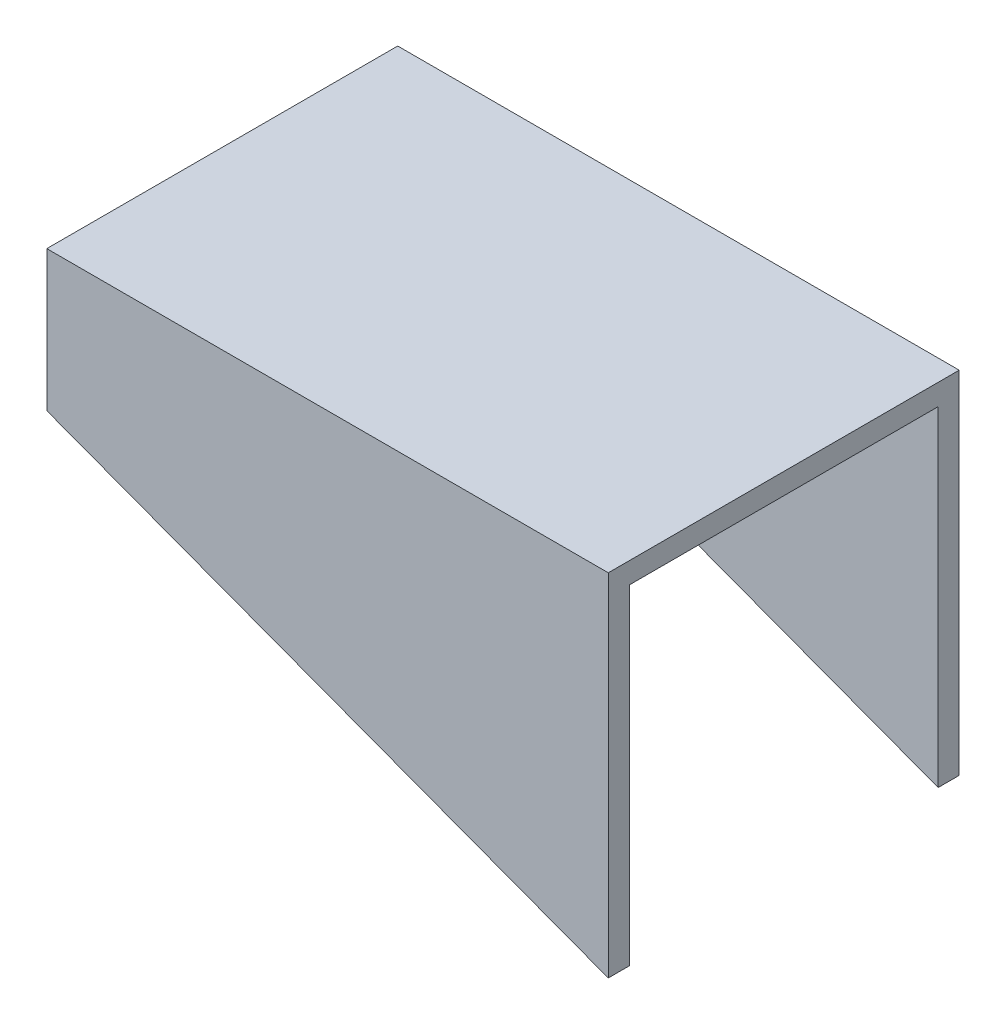
from build123d import *

# Parameters (mm, degrees)
EXTRUDE_1_DEPTH = 50
SHELL_1_T       = -3


with BuildPart() as part:
    # 草图1 → 凸台-拉伸1 (new body)
    with BuildSketch(Plane.XY):
        Polygon((0, 0), (0, 50), (-80, 50), (-80, 30), align=None)
    extrude(amount=EXTRUDE_1_DEPTH)

    # 抽壳1
    shell_1_openings = [part.faces().sort_by_distance(p)[0] for p in [
        (-80, 40, 25),
        (0, 25, 25),
        (-40, 15, 25),
    ]]
    offset(amount=SHELL_1_T, openings=shell_1_openings, kind=Kind.INTERSECTION)


solid = part.part
